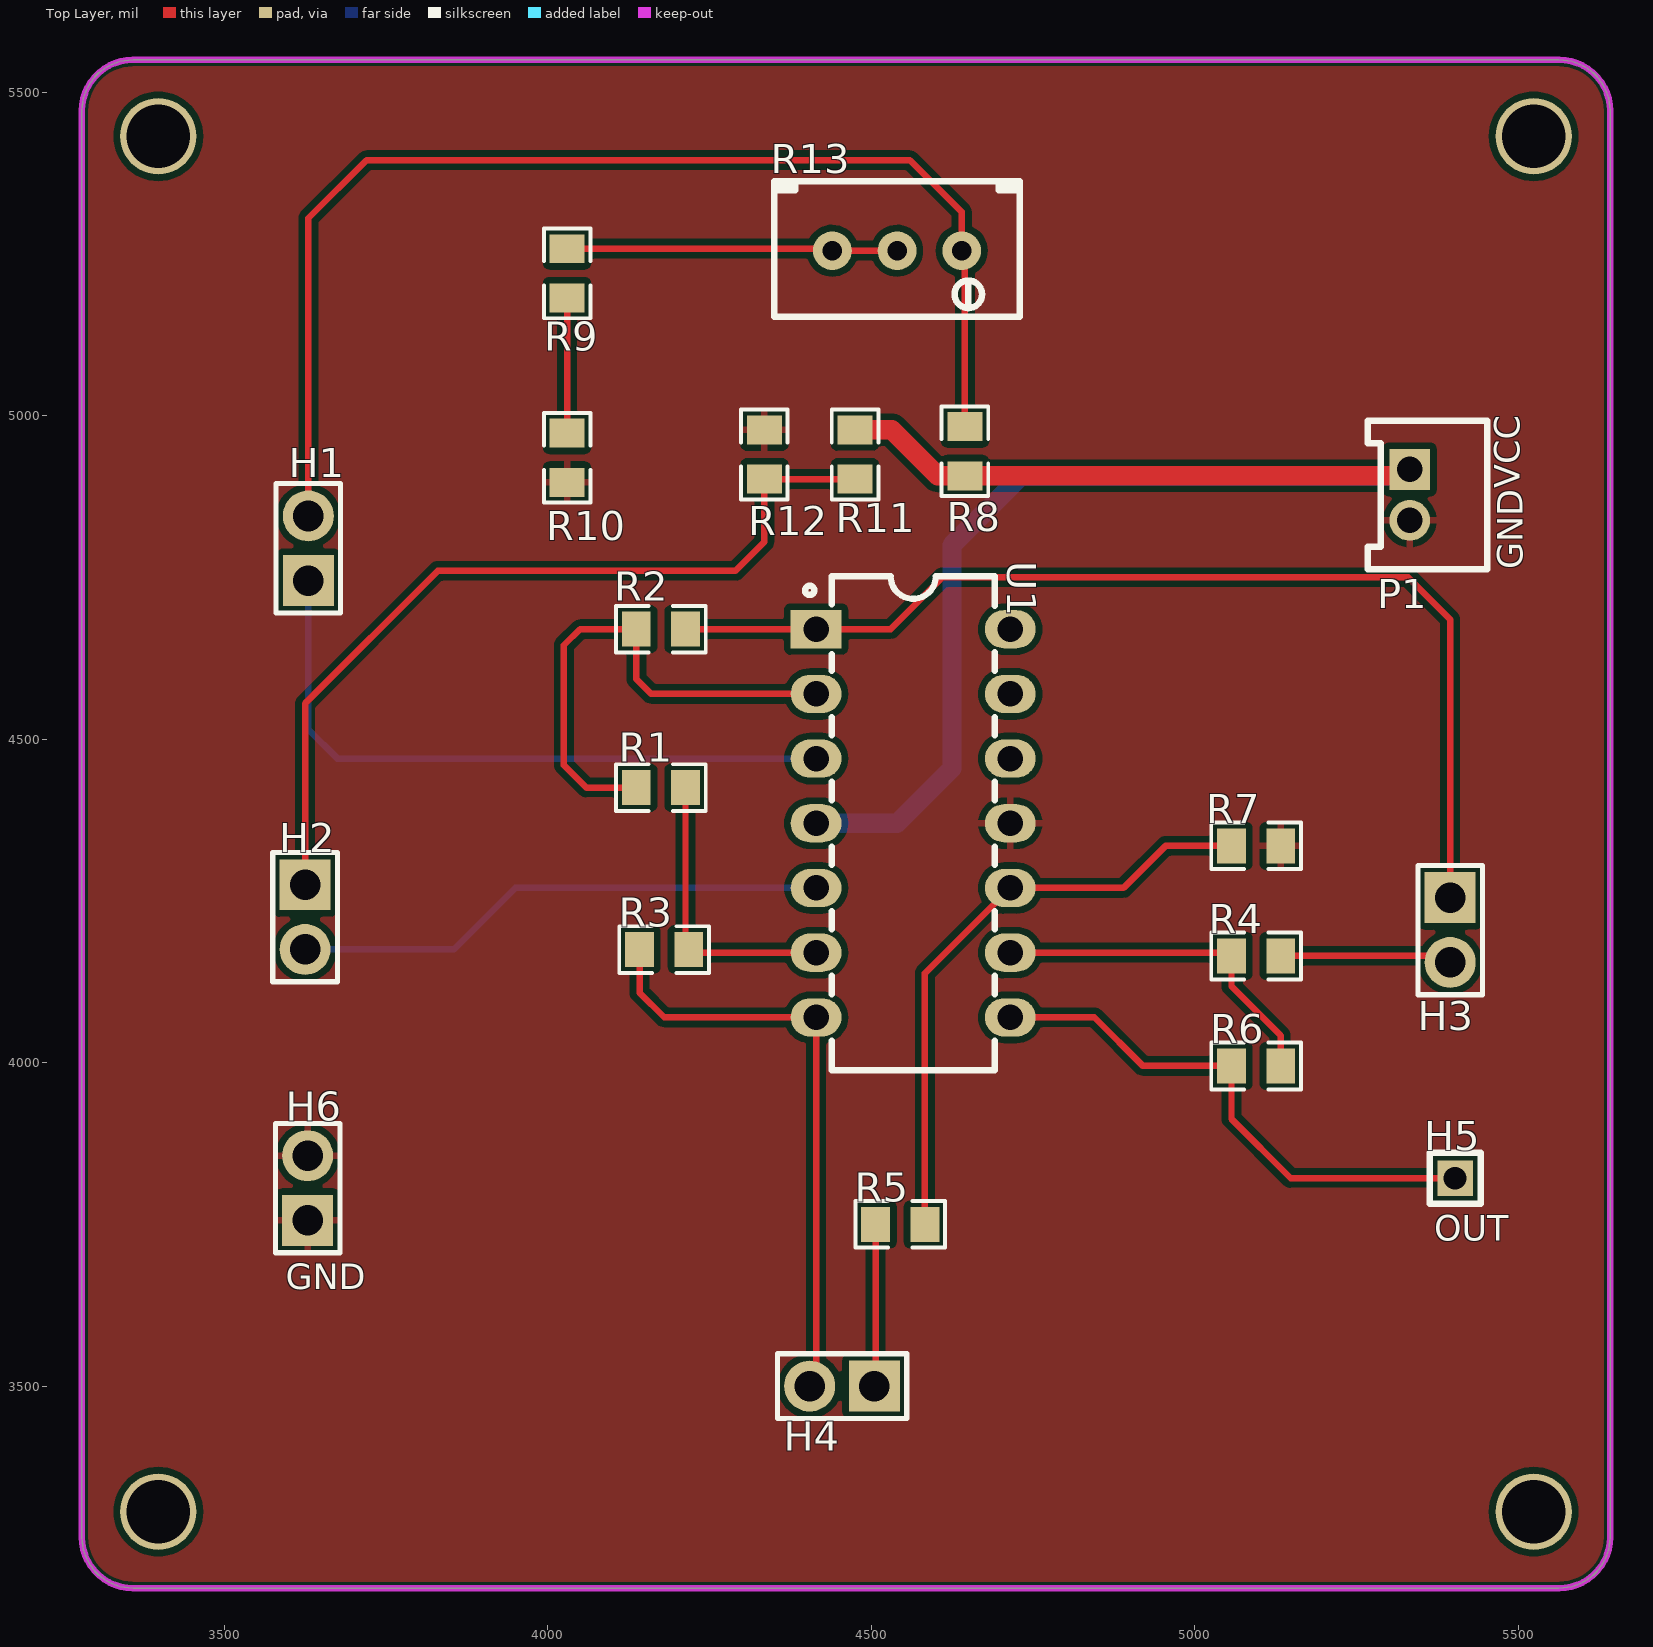
[diagram p0: Top Layer view]
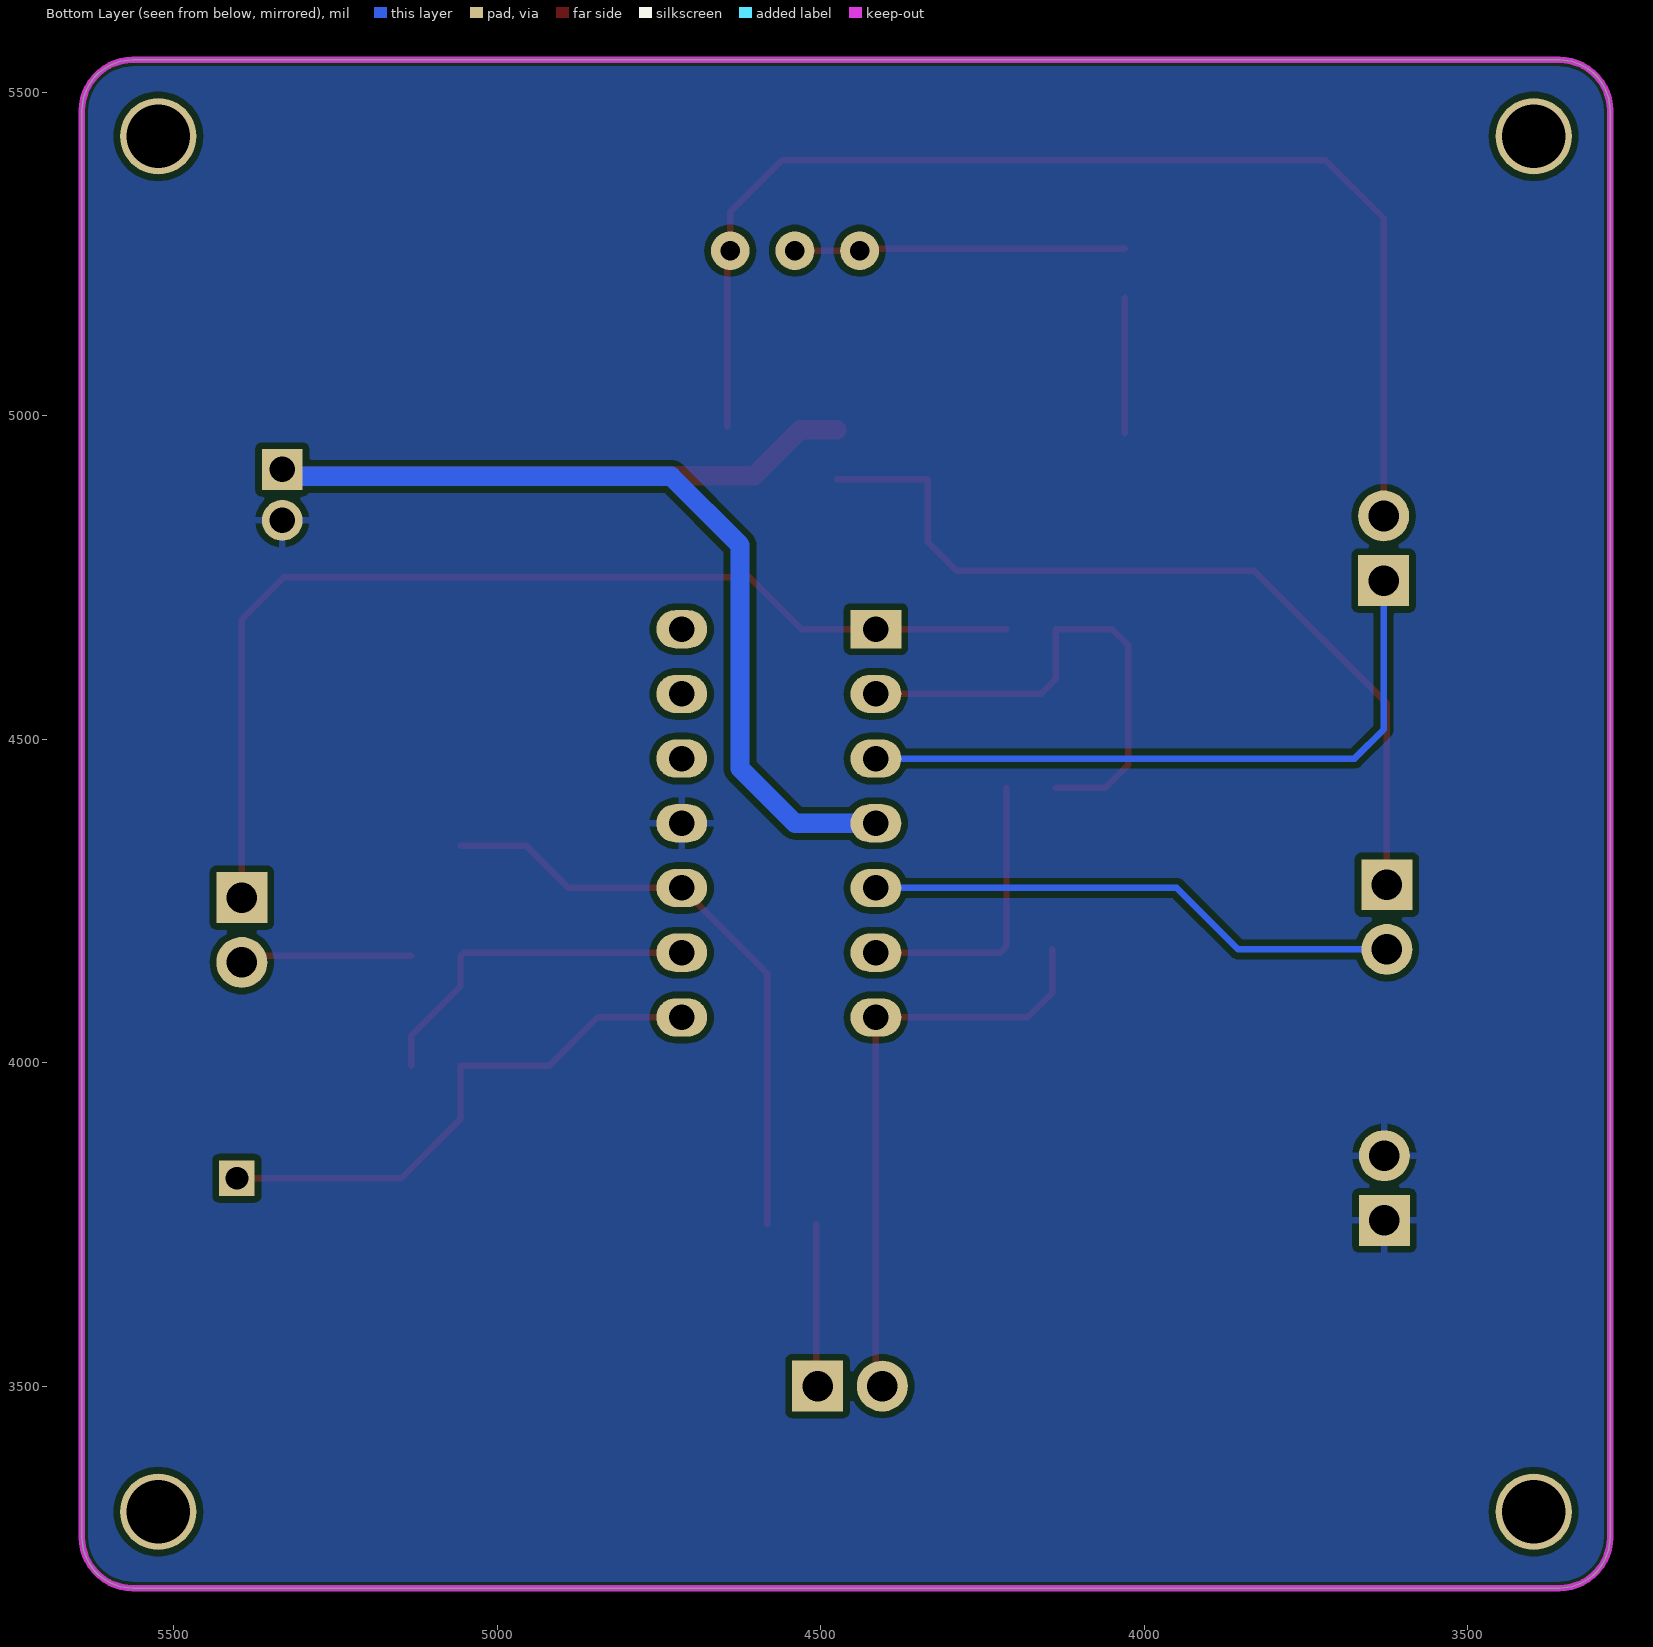
[diagram p1: Bottom Layer view, seen from below]
# Altium PCB MISC89092.pcbdoc
Units mil, origin at the board's own origin, x right, y up, seen from the top; angles counter-clockwise.
Board outline 2362.2 x 2362.2 mil, 2 copper layers (Top Layer, Bottom Layer), stack 62.206 mil thick; 21 components, 17 nets, 58 pads, 0 vias.

## Layer stack, top to bottom
Top Solder Mask Layer: solder mask 0.394, Dk 3.3
Top Layer: signal copper 1.379
Dielectric1: surface 59.449, FR4, Dk 4.5
Bottom Layer: signal copper 1.378
Bottom Solder Mask Layer: solder mask 0.394, Dk 3.3

## Board outline
3358.74,5550 ccw(c3358.74,5471.26) 3280,5471.26 3280,3266.54 ccw(c3358.74,3266.54) 3358.74,3187.8 5563.46,3187.8 ccw(c5563.46,3266.54) 5642.2,3266.54 5642.2,5471.26 ccw(c5563.46,5471.26) 5563.46,5550 3358.74,5550

## Design rules (kind name [scope] priority, off if disabled: settings)
BoardOutlineClearance copperThickness2oz_1 [All] p2 off: genericclearance=7.99 ignorepadtopadclearanceinfootprint=FALSE except(0: Arc-SplitContinuation Track-SplitContinuation SMDPad-SplitContinuation THPad-SplitContinuation Via-SplitContinuation Fill-SplitContinuation Region-SplitContinuation Poly-SplitContinuation Text-SplitContinuation Hole-SplitContinuation; 5.98: Arc-CutoutEdge Track-CutoutEdge SMDPad-CutoutEdge THPad-CutoutEdge Via-CutoutEdge Text-CutoutEdge; 6.9: Hole-OutlineEdge Hole-CutoutEdge; 10: Poly-OutlineEdge Poly-CutoutEdge; 11.81: Arc-OutlineEdge Track-OutlineEdge SMDPad-OutlineEdge THPad-OutlineEdge Via-OutlineEdge Fill-OutlineEdge Region-OutlineEdge Text-OutlineEdge Fill-CutoutEdge Region-CutoutEdge)
BoardOutlineClearance Plane_innerPlane_1 [All] p4 off: genericclearance=4.02 ignorepadtopadclearanceinfootprint=FALSE except(0: Arc-SplitContinuation Track-SplitContinuation SMDPad-SplitContinuation THPad-SplitContinuation Via-SplitContinuation Fill-SplitContinuation Region-SplitContinuation Poly-SplitContinuation Text-SplitContinuation Hole-SplitContinuation; 5.98: Arc-CutoutEdge Track-CutoutEdge SMDPad-CutoutEdge THPad-CutoutEdge Via-CutoutEdge Text-CutoutEdge; 6.9: Hole-OutlineEdge Hole-CutoutEdge; 10: Poly-OutlineEdge Poly-CutoutEdge; 11.81: Arc-OutlineEdge Track-OutlineEdge SMDPad-OutlineEdge THPad-OutlineEdge Via-OutlineEdge Fill-OutlineEdge Region-OutlineEdge Text-OutlineEdge Fill-CutoutEdge Region-CutoutEdge)
BoardOutlineClearance Copper_copperRegion_1 [All] p6 off: genericclearance=4.02 ignorepadtopadclearanceinfootprint=FALSE except(0: Arc-SplitContinuation Track-SplitContinuation SMDPad-SplitContinuation THPad-SplitContinuation Via-SplitContinuation Fill-SplitContinuation Region-SplitContinuation Poly-SplitContinuation Text-SplitContinuation Hole-SplitContinuation; 5.98: Arc-CutoutEdge Track-CutoutEdge SMDPad-CutoutEdge THPad-CutoutEdge Via-CutoutEdge Text-CutoutEdge; 6.9: Hole-OutlineEdge Hole-CutoutEdge; 10: Poly-OutlineEdge Poly-CutoutEdge; 11.81: Arc-OutlineEdge Track-OutlineEdge SMDPad-OutlineEdge THPad-OutlineEdge Via-OutlineEdge Fill-OutlineEdge Region-OutlineEdge Text-OutlineEdge Fill-CutoutEdge Region-CutoutEdge)
BoardOutlineClearance copperThickness1oz_1 [All] p8: genericclearance=4.02 ignorepadtopadclearanceinfootprint=FALSE except(0: Arc-SplitContinuation Track-SplitContinuation SMDPad-SplitContinuation THPad-SplitContinuation Via-SplitContinuation Fill-SplitContinuation Region-SplitContinuation Poly-SplitContinuation Text-SplitContinuation Hole-SplitContinuation; 5.98: Arc-CutoutEdge Track-CutoutEdge SMDPad-CutoutEdge THPad-CutoutEdge Via-CutoutEdge Text-CutoutEdge; 6.9: Hole-OutlineEdge Hole-CutoutEdge; 10: Poly-OutlineEdge Poly-CutoutEdge; 11.81: Arc-OutlineEdge Track-OutlineEdge SMDPad-OutlineEdge THPad-OutlineEdge Via-OutlineEdge Fill-OutlineEdge Region-OutlineEdge Text-OutlineEdge Fill-CutoutEdge Region-CutoutEdge)
Clearance copperThickness2oz [All] p1 off: gap=7.99 ignorepadtopadclearanceinfootprint=FALSE except(5.98: SMDPad-Track SMDPad-SMDPad THPad-Track SMDPad-THPad THPad-THPad Track-Via SMDPad-Via THPad-Via Via-Via Fill-SMDPad Region-SMDPad Fill-THPad Region-THPad Fill-Via Region-Via Fill-Fill Fill-Region Region-Region Arc-Track Arc-SMDPad Arc-THPad Arc-Via Fill-Arc Region-Arc Arc-Arc Text-Track SMDPad-Text Text-THPad Text-Via Fill-Text Region-Text Arc-Text Text-Text; 6.9: Hole-Track Hole-SMDPad Hole-THPad Hole-Via Fill-Hole Region-Hole Hole-Arc Hole-Text; 10: Poly-Track Poly-SMDPad Poly-THPad Poly-Via Poly-Fill Poly-Region Poly-Poly Poly-Arc Poly-Text Poly-Hole; 11.81: Fill-Track Region-Track)
Clearance Plane_innerPlane [All] p3 off: gap=4.02 ignorepadtopadclearanceinfootprint=FALSE except(5.98: SMDPad-Track SMDPad-SMDPad THPad-Track SMDPad-THPad THPad-THPad Track-Via SMDPad-Via THPad-Via Via-Via Fill-SMDPad Region-SMDPad Fill-THPad Region-THPad Fill-Via Region-Via Fill-Fill Fill-Region Region-Region Arc-Track Arc-SMDPad Arc-THPad Arc-Via Fill-Arc Region-Arc Arc-Arc Text-Track SMDPad-Text Text-THPad Text-Via Fill-Text Region-Text Arc-Text Text-Text; 6.9: Hole-Track Hole-SMDPad Hole-THPad Hole-Via Fill-Hole Region-Hole Hole-Arc Hole-Text; 10: Poly-Track Poly-SMDPad Poly-THPad Poly-Via Poly-Fill Poly-Region Poly-Poly Poly-Arc Poly-Text Poly-Hole; 11.81: Fill-Track Region-Track)
Clearance Copper_copperRegion [All] p5 off: gap=4.02 ignorepadtopadclearanceinfootprint=FALSE except(5.98: SMDPad-Track SMDPad-SMDPad THPad-Track SMDPad-THPad THPad-THPad Track-Via SMDPad-Via THPad-Via Via-Via Fill-SMDPad Region-SMDPad Fill-THPad Region-THPad Fill-Via Region-Via Fill-Fill Fill-Region Region-Region Arc-Track Arc-SMDPad Arc-THPad Arc-Via Fill-Arc Region-Arc Arc-Arc Text-Track SMDPad-Text Text-THPad Text-Via Fill-Text Region-Text Arc-Text Text-Text; 6.9: Hole-Track Hole-SMDPad Hole-THPad Hole-Via Fill-Hole Region-Hole Hole-Arc Hole-Text; 10: Poly-Track Poly-SMDPad Poly-THPad Poly-Via Poly-Fill Poly-Region Poly-Poly Poly-Arc Poly-Text Poly-Hole; 11.81: Fill-Track Region-Track)
Clearance copperThickness1oz [All] p7: gap=4.02 ignorepadtopadclearanceinfootprint=FALSE except(5.98: SMDPad-Track SMDPad-SMDPad THPad-Track SMDPad-THPad THPad-THPad Track-Via SMDPad-Via THPad-Via Via-Via Fill-SMDPad Region-SMDPad Fill-THPad Region-THPad Fill-Via Region-Via Fill-Fill Fill-Region Region-Region Arc-Track Arc-SMDPad Arc-THPad Arc-Via Fill-Arc Region-Arc Arc-Arc Text-Track SMDPad-Text Text-THPad Text-Via Fill-Text Region-Text Arc-Text Text-Text; 6.9: Hole-Track Hole-SMDPad Hole-THPad Hole-Via Fill-Hole Region-Hole Hole-Arc Hole-Text; 10: Poly-Track Poly-SMDPad Poly-THPad Poly-Via Poly-Fill Poly-Region Poly-Poly Poly-Arc Poly-Text Poly-Hole; 11.81: Fill-Track Region-Track)
DiffPairsRouting differentialPair [All] p1: maxlimit=6 minlimit=6 mostfreqgap=6 toplayer_minwidth=5 toplayer_prefwidth=10 toplayer_maxwidth=100 toplayer_mingap=6 toplayer_prefgap=6 toplayer_maxgap=6 bottomlayer_minwidth=5 bottomlayer_prefwidth=10 bottomlayer_maxwidth=100 bottomlayer_mingap=6 bottomlayer_prefgap=6 bottomlayer_maxgap=6 maxuncoupledlength=10
HoleToHoleClearance otherClearance [All] p1: gap=11.81 allowstackedmicrovias=TRUE
Length netLength [All] p1: minlimit=0 maxlimit=0
PasteMaskExpansion pasteMaskExpansion [All] p1: expansion=0
PlaneConnect innerPlane [All] p1: planeconnectstyle=Relief reliefexpansion=20 reliefentries=4 reliefconductorwidth=10 reliefairgap=10
PolygonConnect copperRegion [All] p1: connectstyle=Relief reliefconductorwidth=10 reliefentries=4 polygonreliefangle="90 Angle" airgapwidth=10 via.connectstyle=Relief via.reliefconductorwidth=10 via.reliefentries=4 via.polygonreliefangle="90 Angle" via.airgapwidth=10
RoutingVias viaSize [All] p1: holewidth=12.01 width=24.02 viastyle="Through Hole" minholewidth=11.81 minwidth=19.68 maxholewidth=248.03 maxwidth=393.7
SolderMaskExpansion solderMaskExpansion [IsVia] p1: expansion=-1000 istentingtop=TRUE
SolderMaskExpansion solderMaskExpansion [All] p2: expansion=2 istentingtop=FALSE
Width copperThickness2oz_2 [All] p1 off: maxlimit=100 minlimit=8 preferedwidth=10
Width copperThickness1oz_2 [All] p2: maxlimit=100 minlimit=5 preferedwidth=10

## Components (designator, comment, footprint, x,y, rotation, side; value= is the part's Value field where it differs from the comment)
H1 "PZ254V-11-02P" HDR-TH_2P-P2.54-V-M 3630,4795 r90 top
H2 "PZ254V-11-02P" HDR-TH_2P-P2.54-V-M 3625,4225 r270 top
H3 "PZ254V-11-02P" HDR-TH_2P-P2.54-V-M 5395,4205 r270 top
H4 "PZ254V-11-02P" HDR-TH_2P-P2.54-V-M 4455,3500 r180 top
H5 "" HDR-TH_1P-V-M_XKB_X4611WV-01I-C28D40 5402.61,3821.39 r270 top
H6 "PZ254V-11-02P" HDR-TH_2P-P2.54-V-M 3629.05,3806.1 r90 top
P1 "PH-2A" CONN-TH_2P-P2.00_PH-2A_C2319 5332.5,4877.5 r90 top
R1 "2K" R0805_1 4175,4425 r180 top
R2 "5K" R0805_1 4175,4670 r0 top
R3 "5K" R0805_1 4180,4175 r0 top
R4 "2K" R0805_1 5095,4165 r0 top
R5 "2K" R0805_1 4545,3750 r180 top
R6 "40K" R0805_1 5095,3995 r0 top
R7 "40K" R0805_1 5095,4335 r180 top
R8 "10K" R0805_1 4645,4945 r270 top
R9 "9.76K" R0805_1 4030,5220 r90 top
R10 "140" R0805_1 4030,4935 r90 top
R11 "10K" R0805_1 4475,4940 r90 top
R12 "10K" R0805_1 4335,4940 r270 top
R13 "100Ω" RES-ADJ-TH_3296W 4540,5255 r270 top
U1 "LM324N" DIP-14_L19.4-W6.4-P2.54-LS7.6-BL 4565,4370 r270 top

## Footprints (in the part's own frame and the unit in brackets; to place one, negate y for a bottom-side part, rotate by r counter-clockwise, add the part's x,y. Pads: shape width x height; smd on the part's side, far side on the other; paste and mask are expansions set on the pad)
CONN-TH_2P-P2.00_PH-2A_C2319 [mm]
  rect 1.6x1.6 hole 1 paste+0 mask+0.051: 1(1,0)
  round 1.6 hole 1 paste+0 mask+0.051: 2(-1,0)
  silkscreen extent -2.92,-3.05 2.92,1.65
DIP-14_L19.4-W6.4-P2.54-LS7.6-BL [mm]
  rect 1.5x2 hole 1: 1(-7.62,-3.811)
  oval 1.5x2 hole 1: 2(-5.08,-3.811) 3(-2.54,-3.811) 4(0,-3.811) 5(2.54,-3.811) 6(5.08,-3.811) 7(7.62,-3.811) 8(7.62,3.811) 9(5.08,3.809) 10(2.54,3.809) 11(0,3.809) 12(-2.54,3.809) 13(-5.08,3.809) 14(-7.62,3.809)
  silkscreen extent -9.7,-4.24 9.7,3.2
HDR-TH_1P-V-M_XKB_X4611WV-01I-C28D40 [mm]
  rect 1.4x1.4 hole 0.9: 1(0,0)
  silkscreen extent -1,-1 1,1
HDR-TH_2P-P2.54-V-M [mm]
  rect 2x2 hole 1.2: 1(-1.27,0)
  round 2 hole 1.2: 2(1.27,0)
  silkscreen extent -2.54,-1.27 2.54,1.27
R0805_1 [mil]
  rect 44.59x54.21 smd: 1(-38.04,0) 2(38.04,0)
  silkscreen extent -69,-36 69,36
RES-ADJ-TH_3296W [mil]
  round 60 hole 30: 1(0,100.01) 2(0,0.01) 3(0,-99.99)
  silkscreen extent -108,-190 102,190

## Free pads (board coordinates)
  round 118.11 hole 98.43: 4(3398.11,3305.91) 4(3398.11,5431.89) 4(5524.09,3305.91) 4(5524.09,5431.89)

## Nets (pads, with @x,y where several pads share a name; then routed paths per layer and width w, separated by ;. In a path a pad name is that pad's centre, name@x,y a point inside that pad or via, vN(x,y) a via of type N, cw(c..) or ccw(c..) an arc to the next point about the centre after c; other vN are vias at no path point)
$1N346: R1.2 R2.1 U1.2 | length 798.3
  Top Layer w10: R1.2 4060,4425 4025,4460 4025,4645 4050,4670 R2.1 4136.96,4593.04 4160,4570 U1.2
$1N351: R1.1 R3.2 U1.6 | length 451.1
  Top Layer w10: R1.1 4213.04,4180 R3.2 4223.04,4170 U1.6
$1N421: H4.2 R3.1 U1.7 | length 929.9
  Top Layer w10: R3.1 4141.96,4108.04 4180,4070 U1.7 4414.98,3509.98 H4.2
$1N436: H3.1 R2.2 U1.1 | length 1672
  Top Layer w10: R2.2 U1.1 4530,4670 4610,4750 5330,4750 5395,4685 H3.1
$1N561: R5.1 R7.2 U1.10 | length 943.6
  Top Layer w10: R5.1 4583.04,4138.06 U1.10 4890,4270 4955,4335 R7.2
$1N570: R4.1 R6.2 U1.9 | length 545.6
  Top Layer w10: U1.9 5051.96,4170 R4.1 5056.96,4118.04 5133.04,4041.96 R6.2
$1N693: H5.1 R6.1 U1.8 | length 838.6
  Top Layer w10: U1.8 4845,4070 4920,3995 R6.1 5056.96,3913.04 5148.6,3821.39 H5.1
$1N835: H4.1 R5.2 | length 250.8
  Top Layer w10: H4.1 4506.96,3501.96 R5.2
$1N850: H3.2 R4.2 | length 266.1
  Top Layer w10: R4.2 5385,4165 H3.2
$1N1237: H2.1 R11.1 R12.2 | length 1330.5
  Top Layer w10: H2.1 3625,4555 3830,4760 4290,4760 4335,4805 R12.2 R11.1
$1N1241: R9.1 R10.2 | length 208.9
  Top Layer w10: R10.2 R9.1
$1N1361: H1.2 R8.1 R13.1 | length 1874.4
  Top Layer w10: H1.2 3630,5305 3720,5395 4560,5395 4640,5315 R13.1 4645,5250 R8.1
$1N1365: R9.2 R13.2 R13.3 | length 511.3
  Top Layer w10: R9.2 4436.96,5258.04 R13.3 R13.2
$1N1384: H1.1 U1.3 | length 1033.6
  Bottom Layer w10: H1.1 3630,4515 3675,4470 U1.3
$1N1398: H2.2 U1.5 | length 829.3
  Bottom Layer w10: H2.2 3855,4175 3950,4270 U1.5
GND: H6.1 H6.2 P1.2 R7.1 R10.1 R12.1 U1.11
VCC: P1.1 R8.2 R11.2 U1.4 | length 2237.2
  Top Layer w30: R11.2 4531.96,4978.04 4603.04,4906.96 R8.2 5322.59,4906.96 P1.1
  Bottom Layer w30: U1.4 4540,4370 4625,4455 4625,4800 4731.21,4906.21 5321.84,4906.21 P1.1
pads on no net: U1.12 U1.13 U1.14

## Polygon pours and split planes (outlines as drawn)
GND on Top Layer (solid, remove dead copper, pour order 0): 3000,5710 3000,3000 5995,3000 5995,5710
GND on Bottom Layer (solid, remove dead copper, pour order 2): 3165,5670 3165,3100 5835,3100 5835,5670

## Keep-outs
Board Outline Layer:
  the board outline again, w10

## Silkscreen, mask and mechanical layers (free items; w line width, h text height)
Top Silkscreen Layer:
  text "VCC" at 5502.5,4887.5 h39.37 r90
  text "GND" at 5507.5,4762.5 h39.37 r90
  text "OUT" at 5370,3725 h39.37
  text "GND" at 3595,3650 h39.37